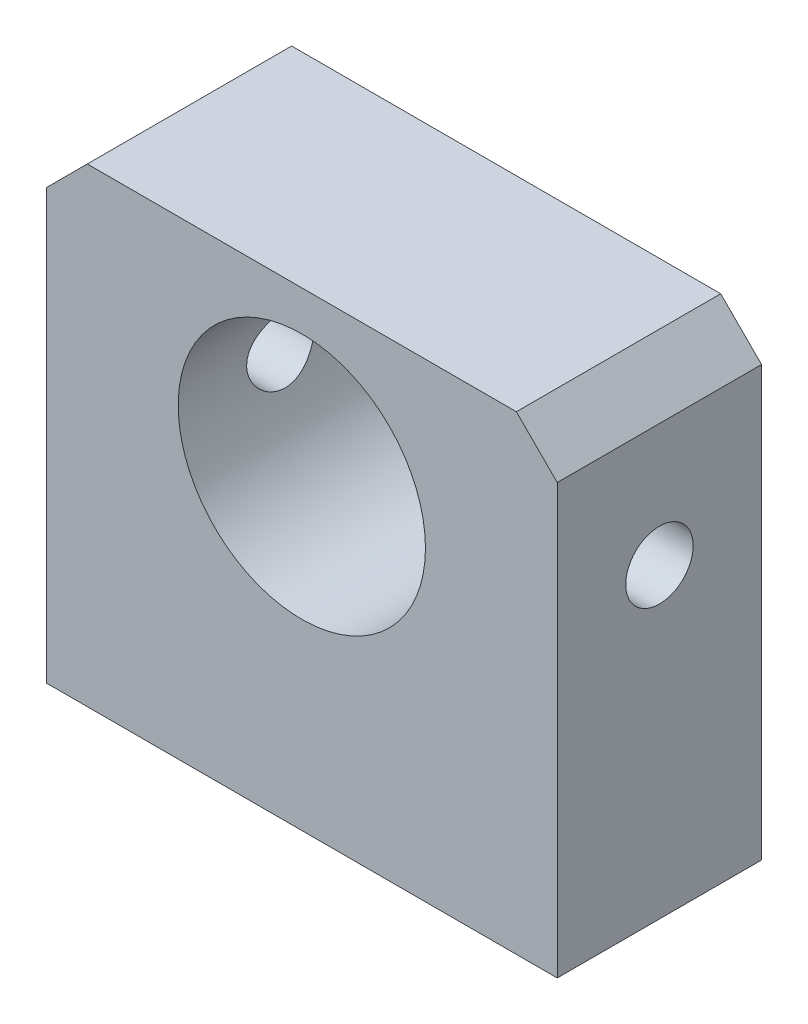
from build123d import *

# Parameters (mm, degrees)
SKETCH1_W             = 25
SKETCH1_H             = 23
BOSS_EXTRUDE1_DEPTH   = 10
SKETCH2_R             = 6.05
CUT_EXTRUDE1_DEPTH    = 20.710403344
CHAMFER1_SIZE         = 2
M4_TAPPED_HOLE1_D     = 3.3
M4_TAPPED_HOLE1_DEPTH = 10.1
M4_TAPPED_HOLE1_TIP   = 0.991420021


with BuildPart() as part:
    # Sketch1 → Boss-Extrude1 (new body)
    with BuildSketch(Plane.XY):
        Rectangle(SKETCH1_W, SKETCH1_H)
    extrude(amount=BOSS_EXTRUDE1_DEPTH)

    # Sketch2 → Cut-Extrude1 (cut, through all)
    with BuildSketch(Plane.XY.offset(10)):
        with Locations((0, 3.5)):
            Circle(SKETCH2_R)
    extrude(amount=-CUT_EXTRUDE1_DEPTH, mode=Mode.SUBTRACT)

    # Chamfer1
    chamfer1_edges = [part.edges().sort_by_distance(p)[0] for p in [
        (-12.5, 11.5, 5),
        (12.5, 11.5, 5),
    ]]
    chamfer(chamfer1_edges, length=CHAMFER1_SIZE)

    # M4 Tapped Hole1
    with Locations(Plane.XZ.offset(11.5)):
        with Locations((-7, 5), (7, 5)):
            Hole(M4_TAPPED_HOLE1_D / 2, depth=M4_TAPPED_HOLE1_DEPTH)
            with Locations((0, 0, -(M4_TAPPED_HOLE1_DEPTH + M4_TAPPED_HOLE1_TIP / 2))):  # 118° drill point
                Cone(0, M4_TAPPED_HOLE1_D / 2, M4_TAPPED_HOLE1_TIP, mode=Mode.SUBTRACT)

    # Sketch5 → M4 Tapped Hole2 (revolve, cut)
    with BuildSketch(Plane(origin=(-12.5, 3.5, 5), x_dir=(0, 0, 1), z_dir=(0, 1, 0))):
        Polygon((0, 0), (0, 11.091420021), (1.65, 10.1), (1.65, 0), align=None)
    m4_tapped_hole2 = revolve(axis=Axis((-18.85, 3.5, 5), (1, 0, 0)), mode=Mode.SUBTRACT)

    # Mirror1: M4 Tapped Hole2 across plane
    add(m4_tapped_hole2.mirror(Plane(origin=(0, 0, 0), x_dir=(0, 0, 1), z_dir=(1, 0, 0))), mode=Mode.SUBTRACT)


solid = part.part
